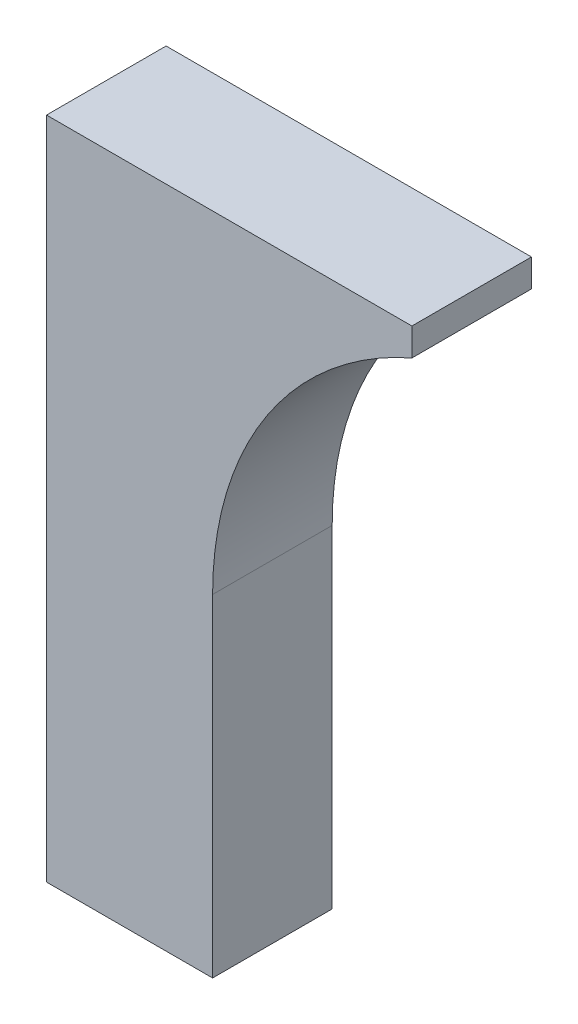
SolidWorks part; units mm, degrees
ref_plane "Front Plane" through (0, 0, 0) normal (0, 0, 1) x (1, 0, 0)
ref_plane "Top Plane" through (0, 0, 0) normal (0, 1, 0) x (1, 0, 0)
ref_plane "Right Plane" through (0, 0, 0) normal (1, 0, 0) x (0, 0, -1)
sketch "Sketch1" plane through (0, 0, 0) normal (0, 0, 1) x (1, 0, 0)
  line L0 (0, 0) -> (0, 100)
  line L1 (0, 100) -> (55, 100)
  line L2 (55, 100) -> (55, 95.8258)
  line L3 (0, 0) -> (25, 0)
  line L4 (25, 0) -> (25, 50)
  arc A0 (55, 95.8258) -> (25, 50) centre (75, 50) ccw
  dimension "D6" = 100
  dimension "D1" = 55
  dimension "D2" = 100
  dimension "D3" = 25
  dimension "D4" = 75
  dimension "D5" = 50
extrude "Boss-Extrude1" add sketch "Sketch1" along normal blind 18
